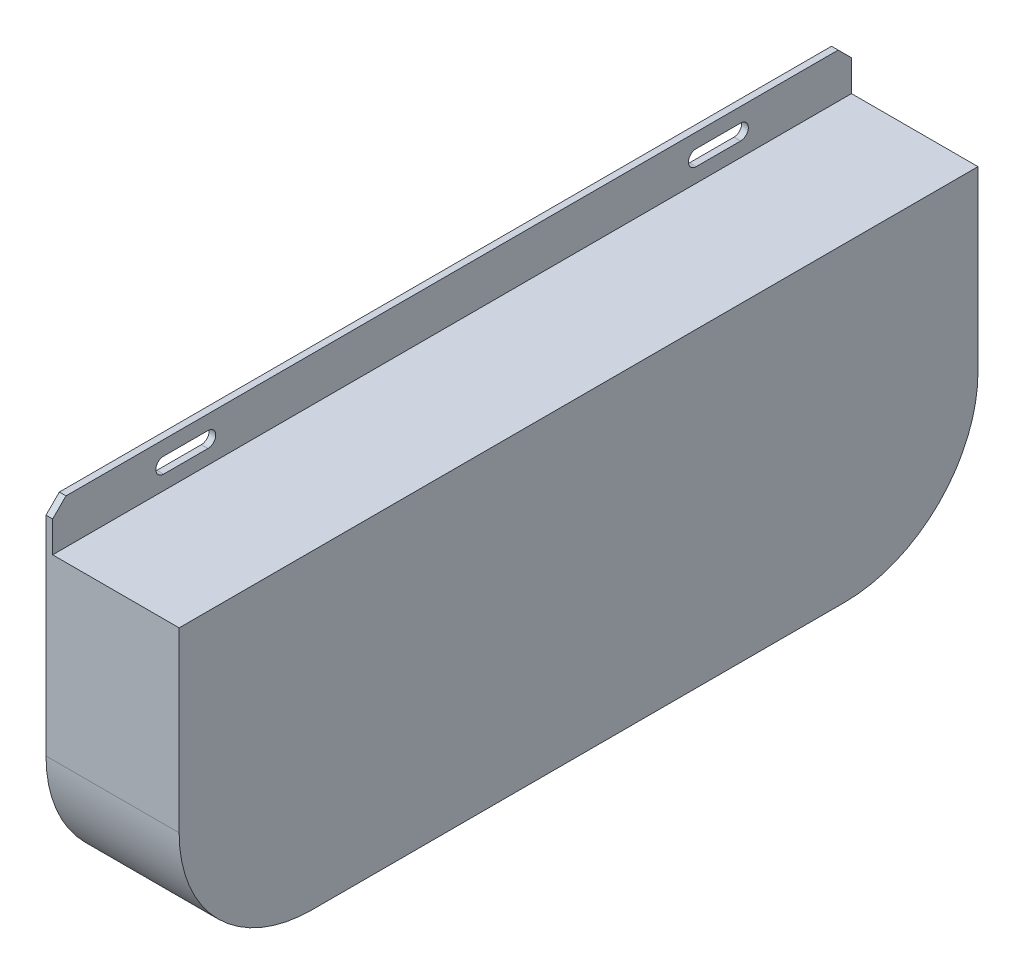
SolidWorks part; units mm, degrees
material "冷轧板 T=1.5mm "
ref_plane "Front" through (0, 0, 0) normal (0, 0, 1) x (1, 0, 0)
ref_plane "Top" through (0, 0, 0) normal (0, 1, 0) x (1, 0, 0)
ref_plane "Right" through (0, 0, 0) normal (1, 0, 0) x (0, 0, -1)
sketch "草图1" plane through (0, 0, 0) normal (1, 0, 0) x (0, 0, -1)
  line L1 (-54.3193, 7.6613) -> (125.6807, 7.6613)
  line L2 (-54.3193, 7.6613) -> (-54.3193, -32.3387)
  line L3 (-24.3193, -62.3387) -> (95.6807, -62.3387)
  line L4 (125.6807, 7.6613) -> (125.6807, -32.3387)
  arc A0 (95.6807, -62.3387) -> (125.6807, -32.3387) centre (95.6807, -32.3387) ccw
  arc A1 (-24.3193, -62.3387) -> (-54.3193, -32.3387) centre (-24.3193, -32.3387) cw
  point P8 (-54.3193, -62.3387)
  dimension "D3" = 30
  dimension "D1" = 180
  dimension "D2" = 70
extrude "凸台-拉伸1" add sketch "草图1" along normal blind 30
shell "抽壳1" thickness 1.5
sketch "草图2" plane through (0, 7.6613, 0) normal (0, 1, 0) x (1, 0, 0)
  line L0 (30, -54.3193) -> (0, -54.3193) construction
  line L1 (0, -54.3193) -> (1.5, -54.3193)
  line L2 (0, -54.3193) -> (0, 125.6807)
  line L3 (0, 125.6807) -> (1.5, 125.6807)
  line L4 (1.5, -54.3193) -> (1.5, 125.6807)
  line L5 (30, 125.6807) -> (0, 125.6807) construction
  line L7 (0, 125.6807) -> (0, -54.3193) construction
  dimension "D2" = 1.5
extrude "凸台-拉伸2" add sketch "草图2" along normal blind 10
sketch "草图5" plane through (0, -62.3387, 0) normal (0, -1, 0) x (1, 0, 0)
  line L1 (0, -25.6807) -> (1.5, -25.6807)
  line L2 (0, -25.6807) -> (0, -45.6807)
  line L3 (0, -45.6807) -> (1.5, -45.6807)
  line L4 (1.5, -25.6807) -> (1.5, -45.6807)
  line L5 (30, -35.6807) -> (1.5, -35.6807) construction
  line L6 (30, 24.3193) -> (30, -95.6807) construction
  line L8 (0, 24.3193) -> (0, -95.6807) construction
  dimension "D1" = 1.5
  dimension "D2" = 20
extrude "凸台-拉伸3" add sketch "草图5" along normal blind 10
sketch "草图4" plane through (1.5, 0, 0) normal (1, 0, 0) x (0, 0, -1)
  line L0 (35.6807, 17.6613) -> (35.6807, -63.0771) construction
  line L1 (-54.3193, 17.6613) -> (125.6807, 17.6613) construction
  line L2 (-29.3193, 12.6613) -> (-19.3193, 12.6613) construction
  line L3 (-29.3193, 14.4113) -> (-19.3193, 14.4113)
  line L4 (-29.3193, 10.9113) -> (-19.3193, 10.9113)
  line L5 (90.6807, 12.6613) -> (100.6807, 12.6613) construction
  line L6 (90.6807, 14.4113) -> (100.6807, 14.4113)
  line L7 (90.6807, 10.9113) -> (100.6807, 10.9113)
  line L8 (30.6807, -67.3387) -> (40.6807, -67.3387) construction
  line L9 (30.6807, -65.5887) -> (40.6807, -65.5887)
  line L10 (30.6807, -69.0887) -> (40.6807, -69.0887)
  line L11 (45.6807, -72.3387) -> (25.6807, -72.3387) construction
  arc A0 (-29.3193, 14.4113) -> (-29.3193, 10.9113) centre (-29.3193, 12.6613) ccw
  arc A1 (-19.3193, 10.9113) -> (-19.3193, 14.4113) centre (-19.3193, 12.6613) ccw
  arc A2 (90.6807, 14.4113) -> (90.6807, 10.9113) centre (90.6807, 12.6613) ccw
  arc A3 (100.6807, 10.9113) -> (100.6807, 14.4113) centre (100.6807, 12.6613) ccw
  arc A4 (30.6807, -65.5887) -> (30.6807, -69.0887) centre (30.6807, -67.3387) ccw
  arc A5 (40.6807, -69.0887) -> (40.6807, -65.5887) centre (40.6807, -67.3387) ccw
  point P6 (-24.3193, 12.6613)
  point P11 (95.6807, 12.6613)
  point P20 (35.6807, -67.3387)
  dimension "D1" = 120
  dimension "D2" = 5
  dimension "D3" = 10
  dimension "D4" = 3.5
  dimension "D5" = 5
extrude "切除-拉伸2" cut sketch "草图4" against normal through all
chamfer "倒角1" distance 3 angle 45 2 edges at (0.75, 17.6613, -125.6807) (0.75, 17.6613, 54.3193)
chamfer "倒角2" distance 3 angle 45 2 edges at (0.75, -72.3387, -25.6807) (0.75, -72.3387, -45.6807)
